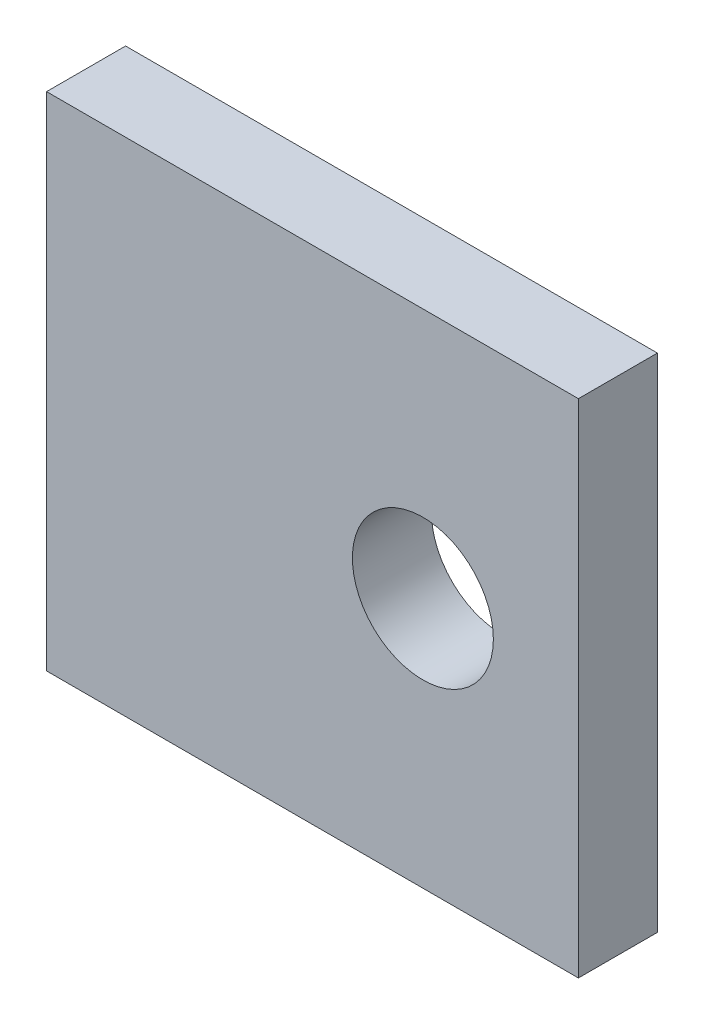
from build123d import *

# Parameters (mm, degrees)
SKETCH1_W           = 53.848
SKETCH1_H           = 50.8
SKETCH1_R           = 7.1374
BOSS_EXTRUDE1_DEPTH = 4


with BuildPart() as part:
    # Sketch1 → Boss-Extrude1 (new, symmetric)
    with BuildSketch(Plane.XY):
        with Locations((-11.176, 0)):
            Rectangle(SKETCH1_W, SKETCH1_H)
        Circle(SKETCH1_R, mode=Mode.SUBTRACT)
    extrude(amount=BOSS_EXTRUDE1_DEPTH, both=True)


solid = part.part
